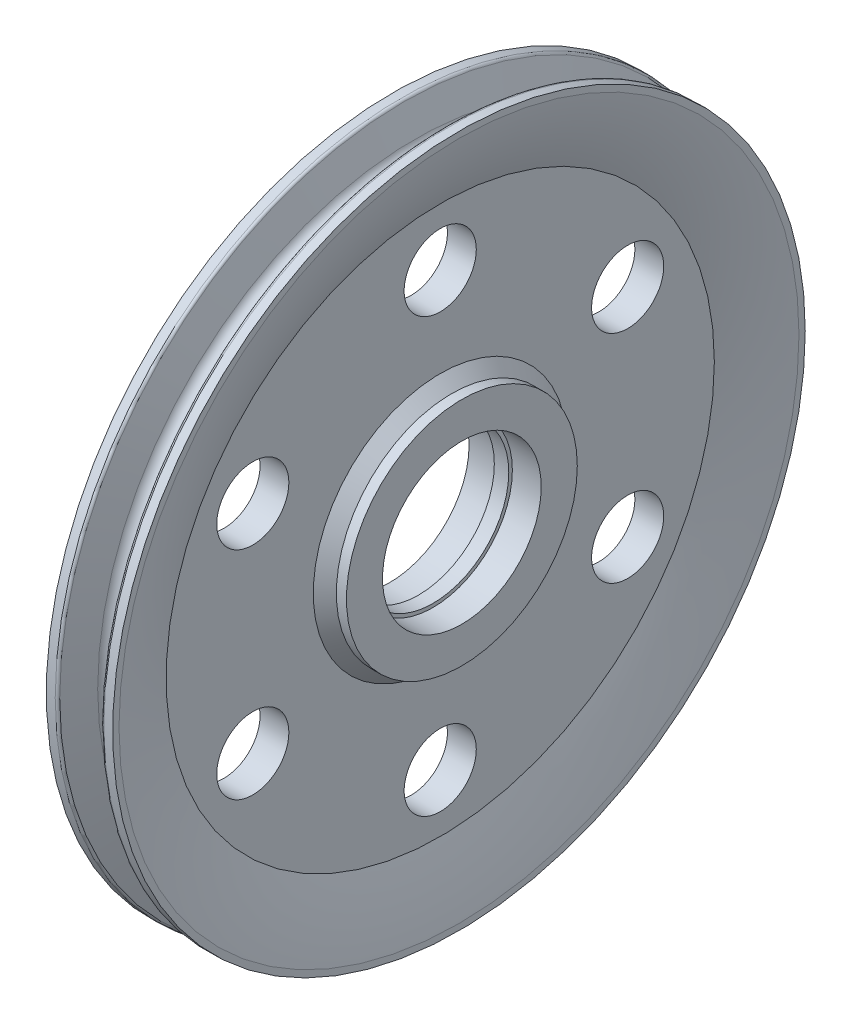
from build123d import *

# Parameters (mm, degrees)
CUT_EXTRUDE1_REACH = 345.074
SKETCH2_R          = 52.5
SKETCH2_R_2        = 25
SKETCH4_R          = 55
CUT_EXTRUDE2_DEPTH = 20
CHAMFER1_SIZE      = 8
FILLET1_R          = 2


with BuildPart() as part:
    # Sketch1 → Revolve1 (revolve)
    with BuildSketch(Plane.XY, mode=Mode.PRIVATE) as revolve1_sk:
        with BuildLine():
            Line((25, 0), (25, 80))
            Line((25, 80), (10, 80))
            Line((10, 80), (10, 190))
            ThreePointArc((10, 190), (17.859035688, 212.437979979), (23, 235.65))
            Line((23, 235.65), (23, 240))
            Line((23, 240), (15.496723781, 240))
            Line((15.496723781, 240), (7.417470837, 220.003147253))
            ThreePointArc((7.417470837, 220.003147253), (0, 215), (-7.417470837, 220.003147253))
            Line((-7.417470837, 220.003147253), (-15.496723781, 240))
            Line((-15.496723781, 240), (-23, 240))
            Line((-23, 240), (-23, 235.65))
            ThreePointArc((-23, 235.65), (-17.859035688, 212.437979979), (-10, 190))
            Line((-10, 190), (-10, 80))
            Line((-10, 80), (-25, 80))
            Line((-25, 80), (-25, 0))
            Line((-25, 0), (25, 0))
        make_face()
    revolve(revolve1_sk.sketch.rotate(Axis((25, 0, 0), (-1, 0, 0)), 90), axis=Axis((25, 0, 0), (-1, 0, 0)))

    # Sketch2 → Cut-Extrude1 (cut, up to next)
    with BuildSketch(Plane(origin=(25, 0, 0), x_dir=(0, 0, -1), z_dir=(1, 0, 0)), mode=Mode.PRIVATE) as cut_extrude1_sk1:
        Circle(SKETCH2_R)
    cut_extrude1_tool1 = extrude(cut_extrude1_sk1.sketch, amount=-CUT_EXTRUDE1_REACH, mode=Mode.PRIVATE) & part.part
    # Sketch2 → Cut-Extrude1 (cut, up to next)
    with BuildSketch(Plane(origin=(25, 0, 0), x_dir=(0, 0, -1), z_dir=(1, 0, 0)), mode=Mode.PRIVATE) as cut_extrude1_sk2:
        with Locations((0, 150)):
            Circle(SKETCH2_R_2)
    cut_extrude1_tool2 = extrude(cut_extrude1_sk2.sketch, amount=-CUT_EXTRUDE1_REACH, mode=Mode.PRIVATE) & part.part
    # Sketch2 → Cut-Extrude1 (cut, up to next)
    with BuildSketch(Plane(origin=(25, 0, 0), x_dir=(0, 0, -1), z_dir=(1, 0, 0)), mode=Mode.PRIVATE) as cut_extrude1_sk3:
        with Locations((129.903810568, 75)):
            Circle(SKETCH2_R_2)
    cut_extrude1_tool3 = extrude(cut_extrude1_sk3.sketch, amount=-CUT_EXTRUDE1_REACH, mode=Mode.PRIVATE) & part.part
    # Sketch2 → Cut-Extrude1 (cut, up to next)
    with BuildSketch(Plane(origin=(25, 0, 0), x_dir=(0, 0, -1), z_dir=(1, 0, 0)), mode=Mode.PRIVATE) as cut_extrude1_sk4:
        with Locations((129.903810568, -75)):
            Circle(SKETCH2_R_2)
    cut_extrude1_tool4 = extrude(cut_extrude1_sk4.sketch, amount=-CUT_EXTRUDE1_REACH, mode=Mode.PRIVATE) & part.part
    # Sketch2 → Cut-Extrude1 (cut, up to next)
    with BuildSketch(Plane(origin=(25, 0, 0), x_dir=(0, 0, -1), z_dir=(1, 0, 0)), mode=Mode.PRIVATE) as cut_extrude1_sk5:
        with Locations((0, -150)):
            Circle(SKETCH2_R_2)
    cut_extrude1_tool5 = extrude(cut_extrude1_sk5.sketch, amount=-CUT_EXTRUDE1_REACH, mode=Mode.PRIVATE) & part.part
    # Sketch2 → Cut-Extrude1 (cut, up to next)
    with BuildSketch(Plane(origin=(25, 0, 0), x_dir=(0, 0, -1), z_dir=(1, 0, 0)), mode=Mode.PRIVATE) as cut_extrude1_sk6:
        with Locations((-129.903810568, -75)):
            Circle(SKETCH2_R_2)
    cut_extrude1_tool6 = extrude(cut_extrude1_sk6.sketch, amount=-CUT_EXTRUDE1_REACH, mode=Mode.PRIVATE) & part.part
    # Sketch2 → Cut-Extrude1 (cut, up to next)
    with BuildSketch(Plane(origin=(25, 0, 0), x_dir=(0, 0, -1), z_dir=(1, 0, 0)), mode=Mode.PRIVATE) as cut_extrude1_sk7:
        with Locations((-129.903810568, 75)):
            Circle(SKETCH2_R_2)
    cut_extrude1_tool7 = extrude(cut_extrude1_sk7.sketch, amount=-CUT_EXTRUDE1_REACH, mode=Mode.PRIVATE) & part.part
    add(cut_extrude1_tool1.solids().sort_by_distance((25, 0, 0))[0], mode=Mode.SUBTRACT)
    add(cut_extrude1_tool2.solids().sort_by_distance((25, 150, 0))[0], mode=Mode.SUBTRACT)
    add(cut_extrude1_tool3.solids().sort_by_distance((25, 75, -129.903811))[0], mode=Mode.SUBTRACT)
    add(cut_extrude1_tool4.solids().sort_by_distance((25, -75, -129.903811))[0], mode=Mode.SUBTRACT)
    add(cut_extrude1_tool5.solids().sort_by_distance((25, -150, 0))[0], mode=Mode.SUBTRACT)
    add(cut_extrude1_tool6.solids().sort_by_distance((25, -75, 129.903811))[0], mode=Mode.SUBTRACT)
    add(cut_extrude1_tool7.solids().sort_by_distance((25, 75, 129.903811))[0], mode=Mode.SUBTRACT)

    # Sketch4 → Cut-Extrude2 (cut)
    with BuildSketch(Plane(origin=(25, 0, 0), x_dir=(0, 0, -1), z_dir=(1, 0, 0))):
        Circle(SKETCH4_R)
    cut_extrude2 = extrude(amount=-CUT_EXTRUDE2_DEPTH, mode=Mode.SUBTRACT)

    # Mirror1: Cut-Extrude2 across plane
    add(cut_extrude2.mirror(Plane(origin=(0, 0, 0), x_dir=(0, 0, 1), z_dir=(1, 0, 0))), mode=Mode.SUBTRACT)

    # Chamfer1
    chamfer1_edges = [part.edges().sort_by_distance(p)[0] for p in [
        (10, 0, 80),
        (-10, 0, 80),
    ]]
    chamfer(chamfer1_edges, length=CHAMFER1_SIZE)

    # Sketch6 → Cut-Revolve1 (revolve, cut)
    with BuildSketch(Plane.XY, mode=Mode.PRIVATE) as cut_revolve1_sk:
        Polygon((-21.329442598, 89.443678278), (3.094493481, 47.140180068), (5.25955699, 48.390180068), (-19.164379089, 90.693678278), align=None)
    revolve(cut_revolve1_sk.sketch.rotate(Axis((-21.329442598, 89.443678278, 0), (0.49999999999999506, -0.8660254037844416, 0)), 180), axis=Axis((-21.329442598, 89.443678278, 0), (0.49999999999999506, -0.8660254037844416, 0)), mode=Mode.SUBTRACT)

    # Fillet1
    fillet1_edges = [part.edges().sort_by_distance(p)[0] for p in [
        (15.496723781, 0, 240),
        (-15.496723781, 0, 240),
    ]]
    fillet(fillet1_edges, radius=FILLET1_R)


solid = part.part
